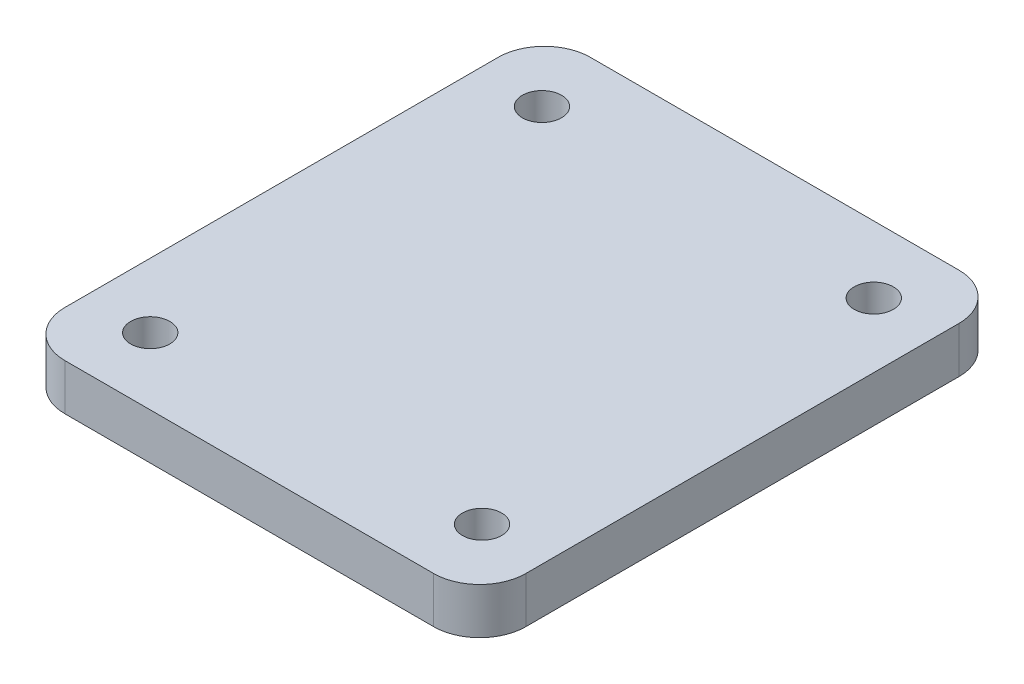
SolidWorks part; units mm, degrees
ref_plane "Front Plane" through (0, 0, 0) normal (0, 0, 1) x (1, 0, 0)
ref_plane "Top Plane" through (0, 0, 0) normal (0, 1, 0) x (1, 0, 0)
ref_plane "Right Plane" through (0, 0, 0) normal (1, 0, 0) x (0, 0, -1)
sketch "Sketch1" plane through (0, 0, 0) normal (0, 1, 0) x (1, 0, 0)
  line L1 (-40, -57) -> (40, -57)
  line L2 (-50, -47) -> (-50, 47)
  line L3 (-40, 57) -> (40, 57)
  line L4 (50, -47) -> (50, 47)
  line L5 (-50, -57) -> (50, 57) construction
  line L6 (-50, 57) -> (50, -57) construction
  line L7 (-36, -42.5) -> (36, -42.5) construction
  line L8 (-36, -42.5) -> (-36, 42.5) construction
  line L9 (-36, 42.5) -> (36, 42.5) construction
  line L10 (36, -42.5) -> (36, 42.5) construction
  line L11 (-36, -42.5) -> (36, 42.5) construction
  line L12 (-36, 42.5) -> (36, -42.5) construction
  arc A0 (-40, -57) -> (-50, -47) centre (-40, -47) cw
  arc A1 (40, -57) -> (50, -47) centre (40, -47) ccw
  arc A2 (40, 57) -> (50, 47) centre (40, 47) cw
  arc A3 (-50, 47) -> (-40, 57) centre (-40, 47) cw
  point P0 (0, 0)
  point P6 (0, 0)
  dimension "D5" = 10
  dimension "D1" = 100
  dimension "D2" = 114
  dimension "D3" = 72
  dimension "D4" = 85
extrude "Boss-Extrude1" add sketch "Sketch1" along normal blind 10
hole_wizard "M10 Tapped Hole1" positions "Sketch3" profile "Sketch4" tap size "M10" standard "GB" end condition through all
sketch "Sketch3" plane through (0, 10, 0) normal (0, 1, 0) x (1, 0, 0)
  line L1 (-36, -42.5) -> (36, -42.5) construction
  line L2 (-36, -42.5) -> (-36, 42.5) construction
  line L3 (-36, 42.5) -> (36, 42.5) construction
  line L4 (36, -42.5) -> (36, 42.5) construction
  line L5 (-36, -42.5) -> (36, 42.5) construction
  line L6 (-36, 42.5) -> (36, -42.5) construction
  point P2 (36, 42.5)
  point P67 (-36, -42.5)
  point P68 (-36, 42.5)
  point P69 (36, -42.5)
  dimension "D1" = 72
  dimension "D2" = 85
  dimension "D3" = 36
  dimension "D4" = 42.5
sketch "Sketch4" plane through (36, 10, -42.5) normal (1, 0, 0) x (0, 0, 1)
  line L0 (0, 0) -> (0, 10)
  line L1 (0, 10) -> (4.25, 10)
  line L2 (4.25, 10) -> (4.25, 0)
  line L5 (4.25, 0) -> (0, 0)
  line L11 (0, -6.35) -> (0, 107.95) construction
  dimension "通孔螺纹孔钻头直径" = 8.5
  dimension "通孔螺纹孔钻头深度" = 10
cosmetic thread "Hole Thread1"
cosmetic thread "Hole Thread2"
cosmetic thread "Hole Thread3"
cosmetic thread "Hole Thread4"
